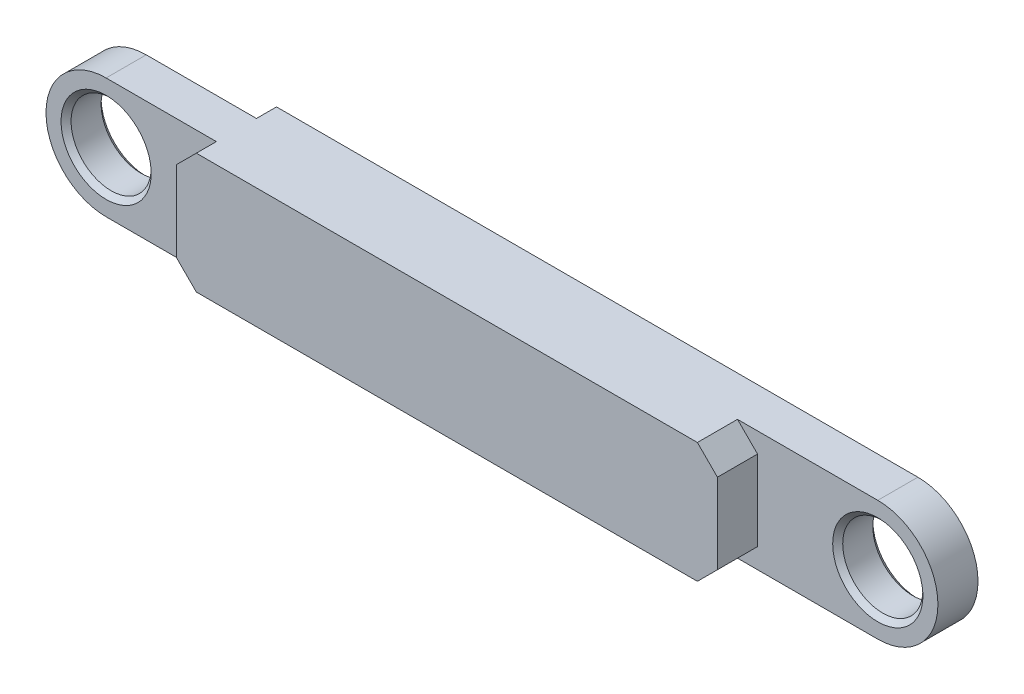
SolidWorks part; units mm, degrees
material "S45C"
ref_plane "Front Plane" through (0, 0, 0) normal (0, 0, 1) x (1, 0, 0)
ref_plane "Top Plane" through (0, 0, 0) normal (0, 1, 0) x (1, 0, 0)
ref_plane "Right Plane" through (0, 0, 0) normal (1, 0, 0) x (0, 0, -1)
sketch "Sketch1" plane through (0, 0, 0) normal (0, 0, 1) x (1, 0, 0)
  line L0 (-37.5, 0) -> (37.5, 0) construction
  line L1 (-37.5, 6) -> (37.5, 6)
  line L2 (-37.5, -6) -> (37.5, -6)
  arc A0 (-37.5, 6) -> (-37.5, -6) centre (-37.5, 0) ccw
  arc A1 (37.5, -6) -> (37.5, 6) centre (37.5, 0) ccw
  point P3 (0, 0)
  dimension "D2" = 6
  dimension "D1" = 75
extrude "Boss-Extrude1" add sketch "Sketch1" along normal mid plane 8
sketch "Sketch2" plane through (0, 0, 4) normal (0, 0, 1) x (1, 0, 0)
  circle A0 centre (37.5, 0) radius 4
  circle A1 centre (-37.5, 0) radius 4
  dimension "D1" = 8
extrude "Cut-Extrude2" cut sketch "Sketch2" against normal through all contours A1
sketch "Sketch3" plane through (0, 6, 0) normal (0, 1, 0) x (1, 0, 0)
  line L0 (37.5, -4) -> (-37.5, -4) construction
  line L1 (25.5, -4) -> (43.5, -4)
  line L2 (25.5, -4) -> (25.5, 0)
  line L3 (25.5, 0) -> (43.5, 0)
  line L4 (43.5, -4) -> (43.5, 0)
  line L5 (43.5, -4) -> (43.5, 4) construction
  line L6 (0, 0) -> (-46.8156, 0) construction
  line L7 (-43.5, -4) -> (-28.5, -4)
  line L8 (-43.5, -4) -> (-43.5, -2)
  line L9 (-43.5, -2) -> (-28.5, -2)
  line L10 (-28.5, -4) -> (-28.5, -2)
  line L11 (-43.5, 4) -> (-28.5, 4)
  line L12 (-43.5, 4) -> (-43.5, 2)
  line L13 (-43.5, 2) -> (-28.5, 2)
  line L14 (-28.5, 4) -> (-28.5, 2)
  line L15 (43.5, 4) -> (37.5, 4) construction
  dimension "D1" = 4
  dimension "D2" = 15
  dimension "D3" = 4
  dimension "D4" = 18
extrude "Cut-Extrude3" cut sketch "Sketch3" against normal through all
chamfer "Chamfer1" distance 2 angle 45 6 edges at (-28.5, 6, -3) (-28.5, -6, -3) (-28.5, 6, 3) (-28.5, -6, 3) (25.5, 6, 2) (25.5, -6, 2)
chamfer "Chamfer2" distance 0.5 angle 45 4 edges at (-33.5, 0, -2) (-41.5, 0, 2) (41.5, 0, -4) (33.5, 0, 0)
